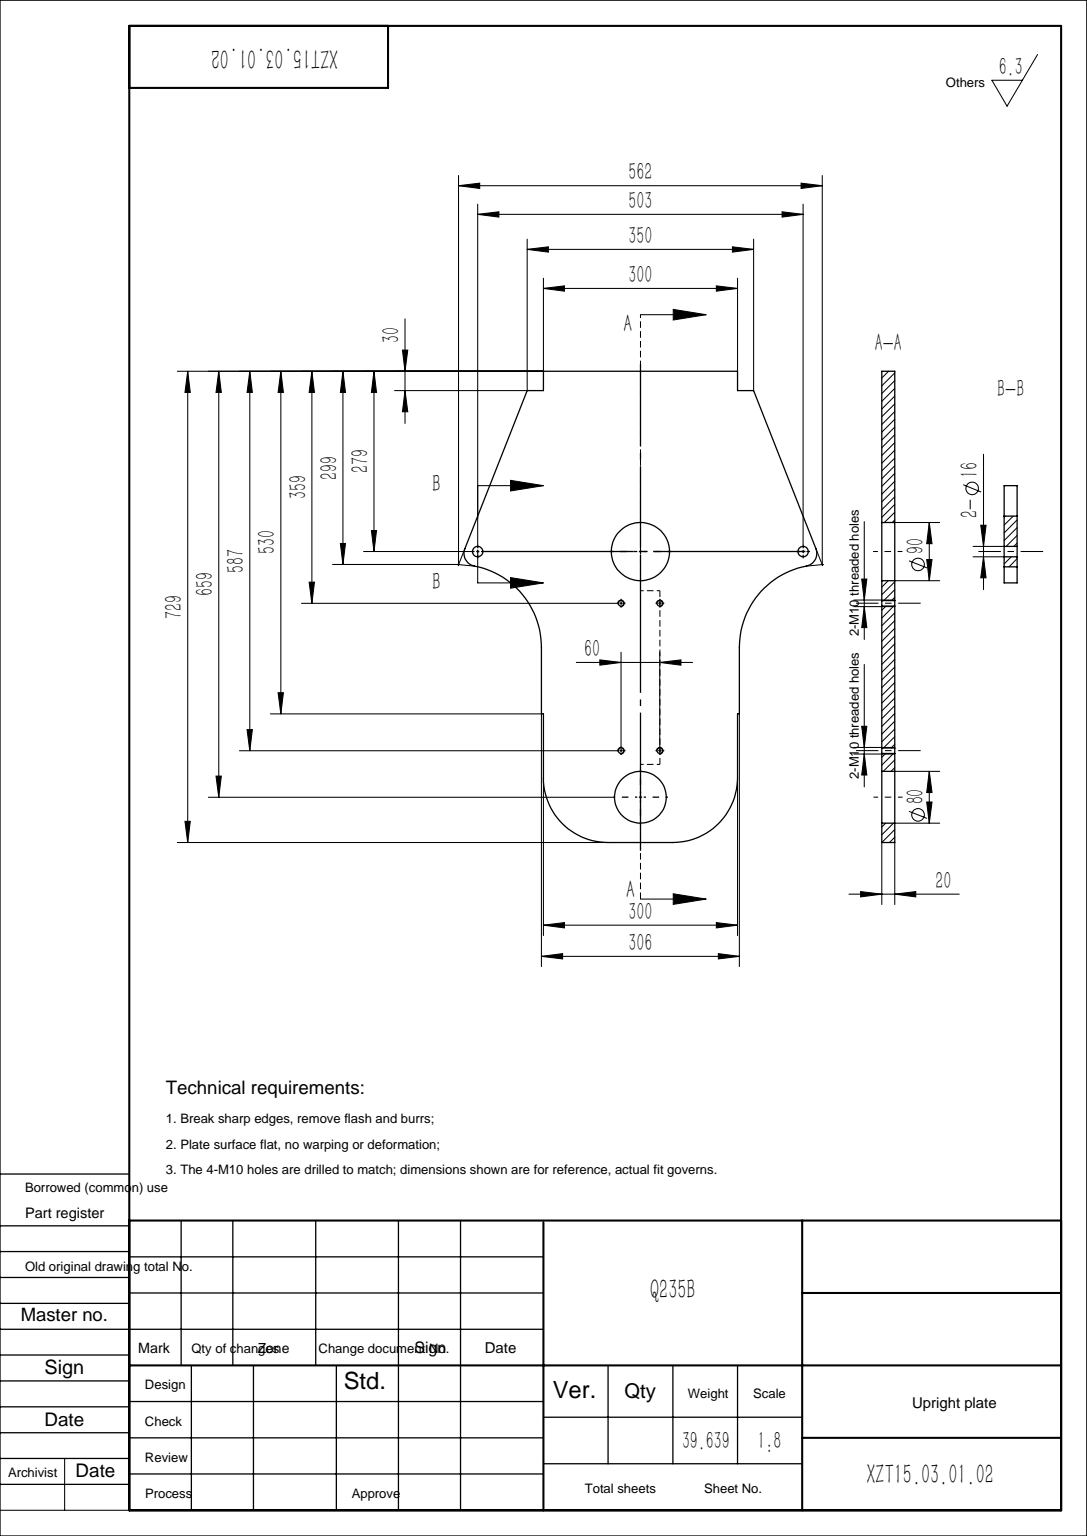
SolidWorks part; units mm, degrees
material "Q235B"
ref_plane "Front Plane" through (0, 0, 0) normal (0, 0, 1) x (1, 0, 0)
ref_plane "Top Plane" through (0, 0, 0) normal (0, 1, 0) x (1, 0, 0)
ref_plane "Right Plane" through (0, 0, 0) normal (1, 0, 0) x (0, 0, -1)
sketch "Sketch1" plane through (0, 0, 0) normal (0, 0, 1) x (1, 0, 0)
  line L0 (-150, 0) -> (150, 0)
  line L1 (150, 0) -> (150, 199)
  line L2 (150, 199) -> (153, 199)
  line L3 (153, 199) -> (153, 302)
  line L5 (281, 430) -> (175, 699)
  line L6 (175, 699) -> (150, 699)
  line L7 (150, 699) -> (150, 729)
  line L8 (150, 729) -> (-150, 729)
  line L9 (0, 729) -> (0, 0) construction
  line L10 (-150, 699) -> (-150, 729)
  line L11 (-175, 699) -> (-150, 699)
  line L12 (-281, 430) -> (-175, 699)
  line L13 (-153, 199) -> (-153, 302)
  line L14 (-150, 199) -> (-153, 199)
  line L15 (-150, 0) -> (-150, 199)
  line L16 (-251.5, 450) -> (0, 450) construction
  arc A0 (153, 302) -> (281, 430) centre (281, 302) cw
  arc A1 (-153, 302) -> (-281, 430) centre (-281, 302) ccw
  circle A2 centre (0, 450) radius 45
  circle A3 centre (0, 70) radius 40
  circle A4 centre (-251.5, 450) radius 8
  circle A6 centre (251.5, 450) radius 8
  dimension "D1" = 300
  dimension "D10" = 80
  dimension "D11" = 90
  dimension "D12" = 279
  dimension "D13" = 16
  dimension "D15" = 659
  dimension "D2" = 306
  dimension "D3" = 300
  dimension "D4" = 350
  dimension "D5" = 562
  dimension "D6" = 30
  dimension "D7" = 729
  dimension "D8" = 299
  dimension "D9" = 530
  dimension "D14" = 503
extrude "Boss-Extrude1" add sketch "Sketch1" along normal blind 20
fillet "Fillet1" radius 100 2 edges at (-150, 0, 10) (150, 0, 10)
fillet "Fillet2" radius 20 2 edges at (-281, 430, 10) (281, 430, 10)
hole_wizard "M10 Tapped Hole1" positions "Sketch2" profile "Sketch3" tap size "M10" standard "GB" end condition up to next
sketch "Sketch2" plane through (0, 0, 20) normal (0, 0, 1) x (1, 0, 0)
  line L0 (0, 0) -> (0, 450) construction
  line L2 (150, 729) -> (-150, 729) construction
  point P0 (-30, 370)
  point P2 (-30, 142)
  point P10 (30, 142)
  point P11 (30, 370)
  dimension "D1" = 60
  dimension "D2" = 359
  dimension "D3" = 587
sketch "Sketch3" plane through (-30, 370, 20) normal (1, 0, 0) x (0, -1, 0)
  line L0 (0, 0) -> (0, 20)
  line L1 (0, 20) -> (4.25, 20)
  line L2 (4.25, 20) -> (4.25, 0)
  line L5 (4.25, 0) -> (0, 0)
  line L11 (0, -6.35) -> (0, 107.95) construction
  dimension "通孔螺纹孔钻头直径" = 8.5
  dimension "通孔螺纹孔钻头深度" = 20
cosmetic thread "CosmeticThread Hole Thread1" parameters "D2"=10
cosmetic thread "CosmeticThread Hole Thread2" parameters "D2"=10
cosmetic thread "CosmeticThread Hole Thread3" parameters "D2"=10
cosmetic thread "CosmeticThread Hole Thread4" parameters "D2"=10
